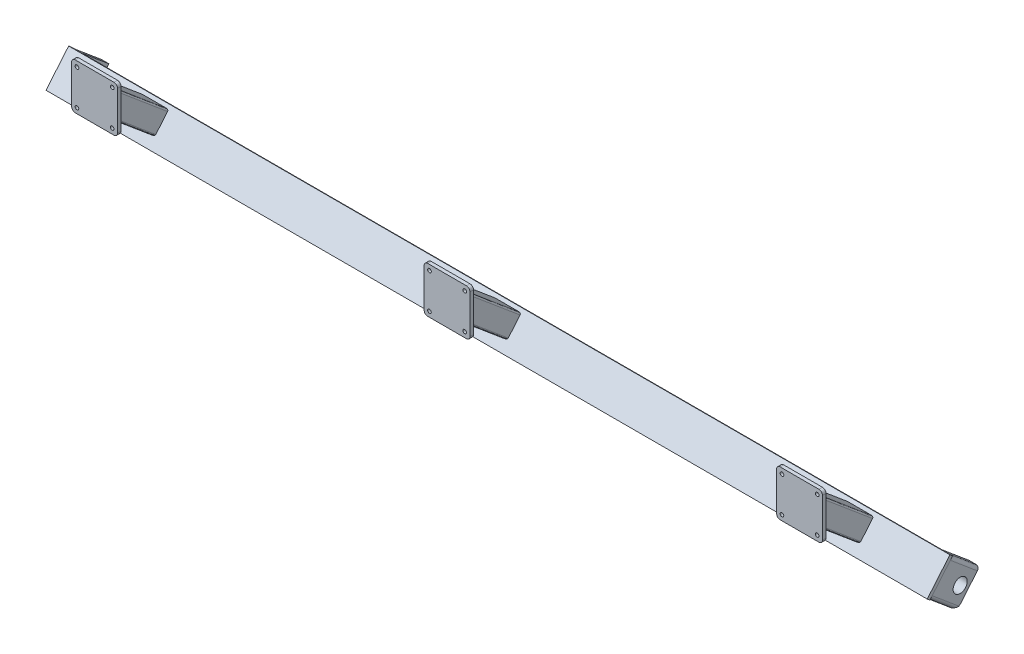
SolidWorks part; units mm, degrees
ref_plane "前视基准面" through (0, 0, 0) normal (0, 0, 1) x (1, 0, 0)
ref_plane "上视基准面" through (0, 0, 0) normal (0, 1, 0) x (1, 0, 0)
ref_plane "右视基准面" through (0, 0, 0) normal (1, 0, 0) x (0, 0, -1)
other "Configuration Table"
sketch "草图1" plane through (0, 0, 0) normal (0, 0, 1) x (1, 0, 0)
  line L1 (-25, 25) -> (25, 25) construction
  line L2 (-25, 25) -> (-25, -25) construction
  line L3 (-25, -25) -> (25, -25) construction
  line L4 (25, 25) -> (25, -25) construction
  line L5 (-25, 25) -> (25, -25) construction
  line L6 (-25, -25) -> (25, 25) construction
  line L7 (-27.5, 32.5) -> (27.5, 32.5)
  line L8 (-32.5, 27.5) -> (-32.5, -27.5)
  line L9 (-27.5, -32.5) -> (27.5, -32.5)
  line L10 (32.5, 27.5) -> (32.5, -27.5)
  line L11 (-32.5, 32.5) -> (32.5, -32.5) construction
  line L12 (-32.5, -32.5) -> (32.5, 32.5) construction
  circle A0 centre (-25, 25) radius 2.6
  circle A1 centre (25, 25) radius 2.6
  circle A2 centre (25, -25) radius 2.6
  circle A3 centre (-25, -25) radius 2.6
  arc A4 (-32.5, -27.5) -> (-27.5, -32.5) centre (-27.5, -27.5) ccw
  arc A5 (27.5, -32.5) -> (32.5, -27.5) centre (27.5, -27.5) ccw
  arc A6 (27.5, 32.5) -> (32.5, 27.5) centre (27.5, 27.5) cw
  arc A7 (-27.5, 32.5) -> (-32.5, 27.5) centre (-27.5, 27.5) ccw
  point P0 (0, 0)
  point P10 (0, 0)
  dimension "D3" = 5.2
  dimension "D6" = 5
  dimension "D1" = 50
  dimension "D2" = 50
  dimension "D4" = 65
  dimension "D5" = 65
extrude "凸台-拉伸1" add sketch "草图1" along normal mid plane 5
sketch "草图2" plane through (0, 0, 0) normal (1, 0, 0) x (0, 0, -1)
  line L0 (2.5, 0) -> (82.5, -67.128)
  line L1 (2.5, -27.5) -> (2.5, 27.5) construction
  dimension "D1" = 80
  dimension "D2" = 50
sketch "草图4" plane through (0, 0, -2.5) normal (0, 0, -1) x (-1, 0, 0)
  line B0 (-18, -17) -> (-18, 17)
  line B1 (17, -20) -> (-17, -20)
  line B2 (20, -17) -> (20, 17)
  line B3 (17, 20) -> (-17, 20)
  line B4 (-20, -17) -> (-20, 17)
  line B5 (20, -20) -> (-20, 20) construction
  line B6 (20, 20) -> (-20, -20) construction
  line B7 (17, 18) -> (-17, 18)
  line B8 (18, -17) -> (18, 17)
  line B9 (17, -18) -> (-17, -18)
  arc B10 (20, 17) -> (17, 20) centre (17, 17) ccw
  arc B11 (17, -20) -> (20, -17) centre (17, -17) ccw
  arc B12 (-17, -20) -> (-20, -17) centre (-17, -17) cw
  arc B13 (-17, 20) -> (-20, 17) centre (-17, 17) ccw
  arc B14 (-17, 18) -> (-18, 17) centre (-17, 17) ccw
  arc B15 (18, 17) -> (17, 18) centre (17, 17) ccw
  arc B16 (17, -18) -> (18, -17) centre (17, -17) ccw
  arc B17 (-17, -18) -> (-18, -17) centre (-17, -17) cw
sketch_block_instance "方管4040-1"
sketch_block "块1" parameters "D2"=3, "D1"=40
sweep "扫描1" add profiles "草图4" path "草图2"
sketch "草图8" plane through (20, 0, 0) normal (1, 0, 0) x (0, 0, -1)
  line L0 (82.5, -47.128) -> (62.8038, -70.6009)
  line L1 (2.5, -20) -> (82.5, -87.128) construction
  line L2 (62.8038, -70.6009) -> (82.5, -87.128)
  line L3 (82.5, -87.128) -> (102.5768, -63.2014)
  line L4 (102.5768, -63.2014) -> (82.5, -47.128)
extrude "切除-拉伸1" cut sketch "草图8" against normal up to surface (40 mm away) up to face at (-20, -33.564, -42.5)
sketch "草图6" plane through (0, -11.0259, -112.7933) normal (0, -0.6428, -0.766) x (-1, 0, 0)
  line L0 (0, -42.128) -> (0, -92.128) construction
  line L1 (-100, -42.128) -> (100, -42.128) construction
  line L2 (-100, -42.128) -> (-100, -92.128) construction
  line L3 (-100, -92.128) -> (100, -92.128) construction
  line L4 (100, -42.128) -> (100, -92.128) construction
  line L6 (-625, -42.128) -> (625, -42.128)
  line L7 (-625, -42.128) -> (-625, -92.128)
  line L8 (-625, -92.128) -> (625, -92.128)
  line L9 (625, -42.128) -> (625, -92.128)
  line L10 (-625, -42.128) -> (625, -92.128) construction
  line L11 (-625, -92.128) -> (625, -42.128) construction
  point P7 (0, -67.128)
  dimension "D1" = 1250
extrude "凸台-拉伸2" add sketch "草图6" along normal blind 5 separate body
sketch "草图7" plane through (0, -63.3094, -75.4492) normal (0, -0.6428, -0.766) x (-1, 0, 0)
  line L3 (-625, -28.0721) -> (625, -28.0721) construction
  line L8 (-620, 21.9279) -> (-610, 21.9279)
  line L17 (-625, 16.9279) -> (-625, -23.0721)
  line L18 (-620, -28.0721) -> (-610, -28.0721)
  line L19 (-610, 21.9279) -> (-610, -28.0721)
  line L21 (620, 21.9279) -> (610, 21.9279)
  line L22 (625, 16.9279) -> (625, -23.0721)
  line L23 (620, -28.0721) -> (610, -28.0721)
  line L24 (610, 21.9279) -> (610, -28.0721)
  arc A6 (625, -23.0721) -> (620, -28.0721) centre (620, -23.0721) cw
  arc A7 (620, 21.9279) -> (625, 16.9279) centre (620, 16.9279) cw
  arc A8 (-625, -23.0721) -> (-620, -28.0721) centre (-620, -23.0721) ccw
  arc A9 (-620, 21.9279) -> (-625, 16.9279) centre (-620, 16.9279) ccw
  point P14 (625, 21.9279)
  point P19 (-625, 21.9279)
  dimension "D3" = 5
  dimension "D1" = 15
  dimension "D2" = 15
extrude "凸台-拉伸3" add sketch "草图7" along normal blind 50 separate body
sketch "草图9" plane through (610, 0, 0) normal (-1, 0, 0) x (0, 0, 1)
  line L0 (-111.7767, -97.8022) -> (-73.4745, -65.6628) construction
  line L1 (-95.707, -116.9533) -> (-127.8464, -78.6511) construction
  line L2 (-57.4048, -84.8139) -> (-89.5442, -46.5117) construction
  circle A0 centre (-100.286, -88.1604) radius 10
  dimension "D1" = 20
  dimension "D2" = 15
extrude "切除-拉伸2" cut sketch "草图9" against normal up to surface and the other way up to surface
sketch "草图10" plane through (625, 0, 0) normal (1, 0, 0) x (0, 0, -1)
  line L0 (98.9209, -113.1231) -> (91.1423, -113.1231)
  line L1 (95.707, -116.9533) -> (57.4048, -84.8139) construction
  line L2 (91.1423, -113.1231) -> (95.707, -116.9533)
  line L3 (95.707, -116.9533) -> (98.9209, -113.1231)
extrude "切除-拉伸3" cut sketch "草图10" against normal up to surface (1250 mm away)
fillet "圆角1" radius 5 1 edges at (617.5, -113.1231, -98.9209)
fillet "圆角2" radius 5 1 edges at (-617.5, -113.1231, -98.9209)
pattern_linear "阵列(线性)1" count 2 spacing 500 along (1, 0, 0) count 2 spacing 500
